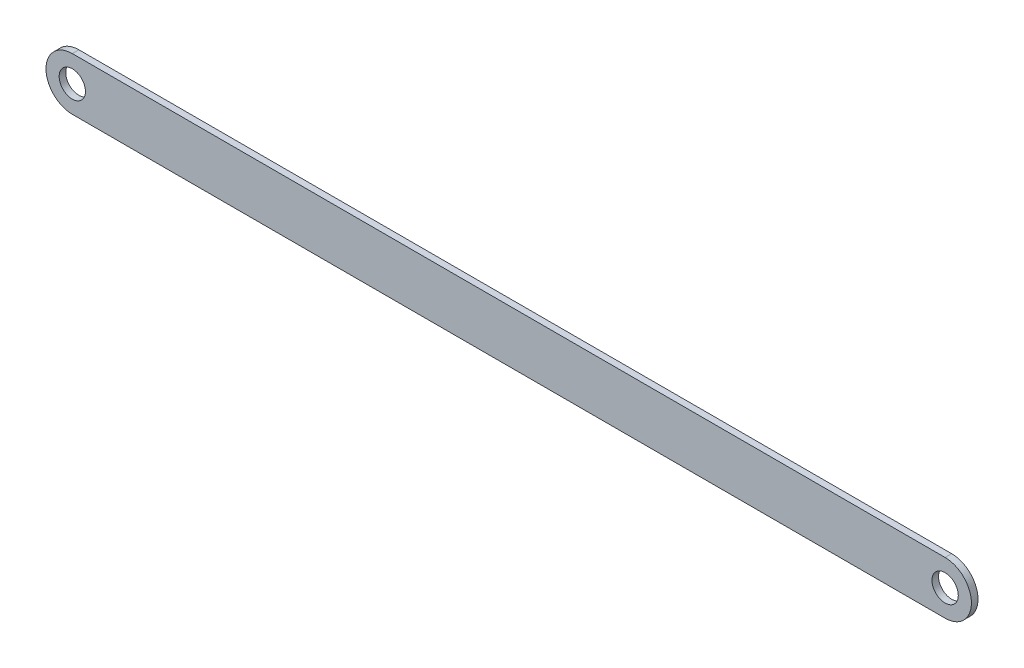
from build123d import *

# Parameters (mm, degrees)
SKETCH1_R           = 5
BOSS_EXTRUDE1_DEPTH = 2.5


with BuildPart() as part:
    # Sketch1 → Boss-Extrude1 (new body)
    with BuildSketch(Plane.XY):
        with BuildLine():
            Line((-165.885, 10), (165.885, 10))
            ThreePointArc((165.885, 10), (175.885, 0), (165.885, -10))
            Line((165.885, -10), (-165.885, -10))
            ThreePointArc((-165.885, -10), (-175.885, 0), (-165.885, 10))
        make_face()
        with Locations((-165.885, 0)):
            Circle(SKETCH1_R, mode=Mode.SUBTRACT)
        with Locations((165.885, 0)):
            Circle(SKETCH1_R, mode=Mode.SUBTRACT)
    extrude(amount=BOSS_EXTRUDE1_DEPTH)


solid = part.part
